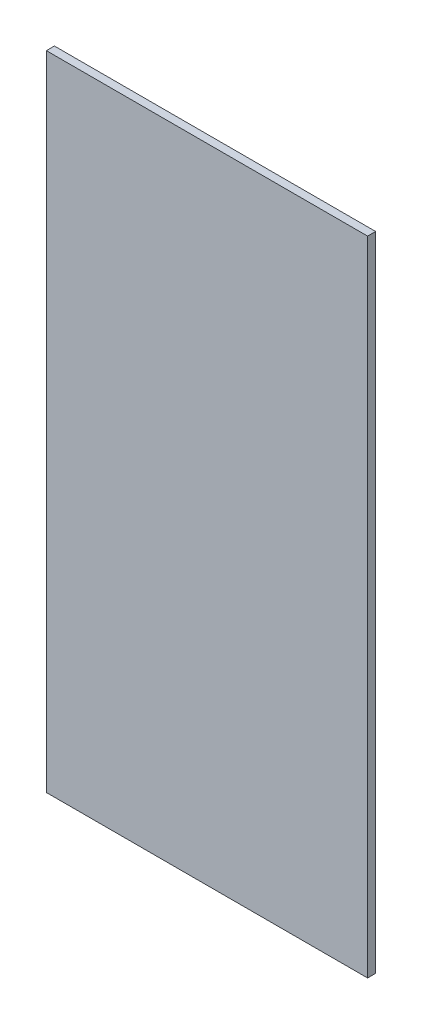
from build123d import *

# Parameters (mm, degrees)
SKETCH_1_W      = 40
SKETCH_1_H      = 80
EXTRUDE_1_DEPTH = 0.5


with BuildPart() as part:
    # 草图1 → 凸台-拉伸1 (new, symmetric)
    with BuildSketch(Plane.XY):
        Rectangle(SKETCH_1_W, SKETCH_1_H)
    extrude(amount=EXTRUDE_1_DEPTH, both=True)


solid = part.part
